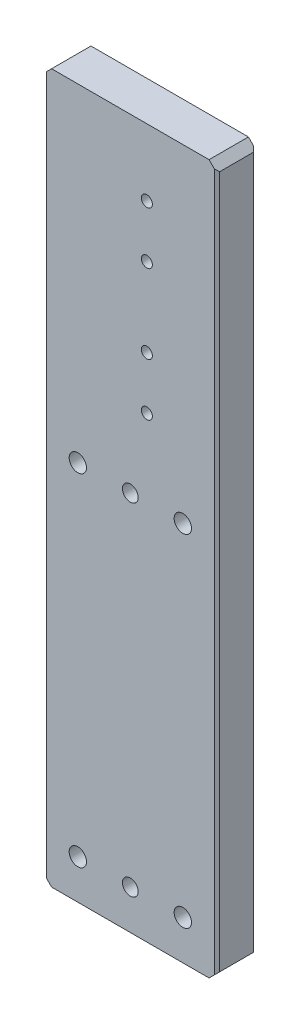
from build123d import *

# Parameters (mm, degrees)
SKETCH1_W                                           = 66
SKETCH1_H                                           = 160
BOSS_EXTRUDE1_DEPTH                                 = 15
CBORE_FOR_M6_HEX_SOCKET_HEAD_CAP_SCREW1_D           = 6.6
CBORE_FOR_M6_HEX_SOCKET_HEAD_CAP_SCREW1_CBORE_D     = 11
CBORE_FOR_M6_HEX_SOCKET_HEAD_CAP_SCREW1_CBORE_DEPTH = 6.4
MOVE_FACE1_BY                                       = 110
M5_TAPPED_HOLE1_D                                   = 4.2
SKETCH6_R                                           = 3.5
CUT_EXTRUDE1_DEPTH                                  = 1.6
CHAMFER2_SIZE                                       = 1
CHAMFER1_SIZE                                       = 3
SKETCH12_R                                          = 3
CUT_EXTRUDE2_DEPTH                                  = 279.354091042


with BuildPart() as part:
    # Sketch1 → Boss-Extrude1 (new body)
    with BuildSketch(Plane.XY):
        with Locations((33, 80)):
            Rectangle(SKETCH1_W, SKETCH1_H)
    extrude(amount=BOSS_EXTRUDE1_DEPTH)

    # CBORE for M6 Hex Socket Head Cap Screw1 (through all)
    with Locations(Plane(origin=(0, 0, 0), x_dir=(-1, 0, 0), z_dir=(0, 0, -1))):
        with Locations((-53, 15), (-13, 15), (-53, 145), (-13, 145)):
            CounterBoreHole(CBORE_FOR_M6_HEX_SOCKET_HEAD_CAP_SCREW1_D / 2, CBORE_FOR_M6_HEX_SOCKET_HEAD_CAP_SCREW1_CBORE_D / 2, CBORE_FOR_M6_HEX_SOCKET_HEAD_CAP_SCREW1_CBORE_DEPTH)

    # Move Face1: a face moved outward by 110.0
    extrude(part.faces().sort_by_distance((33, 160, 7.5))[0], amount=MOVE_FACE1_BY, dir=(0, 1, 0))

    # M5 Tapped Hole1 (through all)
    with Locations(Plane(origin=(0, 0, 0), x_dir=(-1, 0, 0), z_dir=(0, 0, -1))):
        with Locations((-39.3, 244.5), (-39.3, 174.5), (-39.3, 224.5), (-39.3, 194.5)):
            Hole(M5_TAPPED_HOLE1_D / 2)

    # Sketch6 → Cut-Extrude1 (cut)
    with BuildSketch(Plane(origin=(0, 0, 0), x_dir=(-1, 0, 0), z_dir=(0, 0, -1))):
        with Locations((-39.3, 244.5)):
            Circle(SKETCH6_R)
        with Locations((-39.3, 174.5)):
            Circle(SKETCH6_R)
    extrude(amount=-CUT_EXTRUDE1_DEPTH, mode=Mode.SUBTRACT)

    # Chamfer2
    chamfer2_edges = [part.edges().sort_by_distance(p)[0] for p in [
        (66, 135, 15),
        (0, 135, 15),
        (66, 135, 0),
        (0, 135, 0),
    ]]
    chamfer(chamfer2_edges, length=CHAMFER2_SIZE)

    # Chamfer1
    chamfer1_edges = [part.edges().sort_by_distance(p)[0] for p in [
        (0, 0, 7.5),
        (66, 0, 7.5),
        (0, 270, 7.5),
        (66, 270, 7.5),
    ]]
    chamfer(chamfer1_edges, length=CHAMFER1_SIZE)

    # Sketch12 → Cut-Extrude2 (cut, through all)
    with BuildSketch(Plane(origin=(0, 0, 0), x_dir=(-1, 0, 0), z_dir=(0, 0, -1))):
        with Locations((-33, 145)):
            Circle(SKETCH12_R)
        with Locations((-33, 15)):
            Circle(SKETCH12_R)
    extrude(amount=-CUT_EXTRUDE2_DEPTH, mode=Mode.SUBTRACT)


solid = part.part
